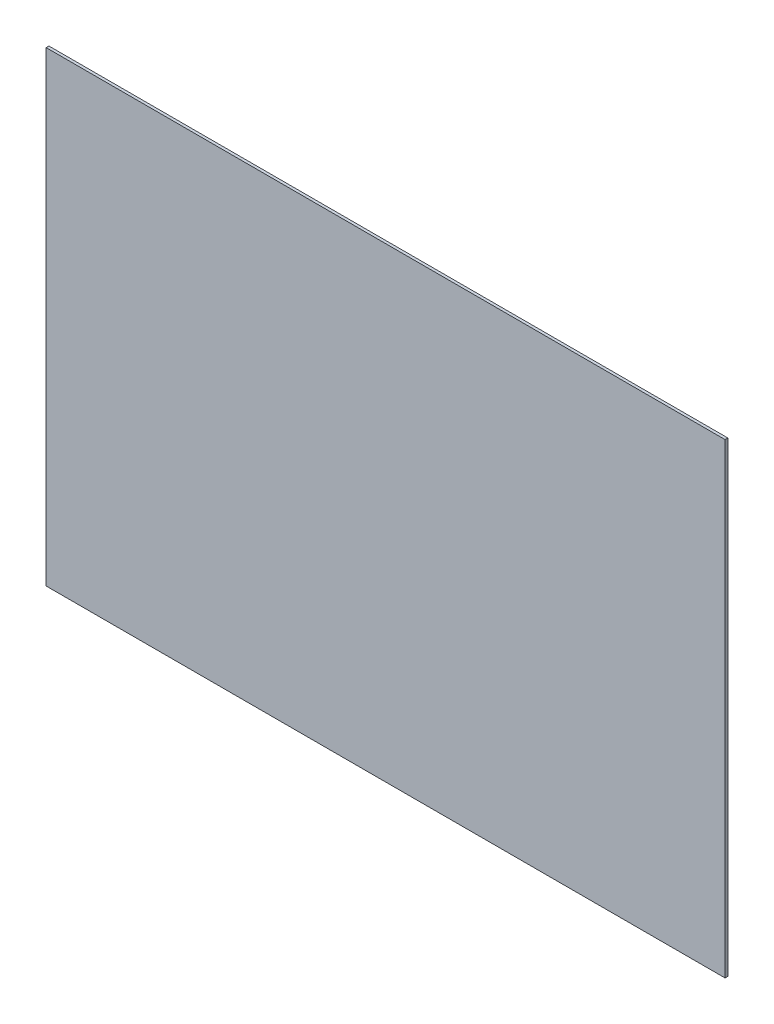
from build123d import *

# Parameters (mm, degrees)
SKETCH_1_W      = 1226
SKETCH_1_H      = 842
EXTRUDE_1_DEPTH = 5


with BuildPart() as part:
    # 草图1 → 凸台-拉伸1 (new body)
    with BuildSketch(Plane.XY):
        Rectangle(SKETCH_1_W, SKETCH_1_H)
    extrude(amount=EXTRUDE_1_DEPTH)


solid = part.part
